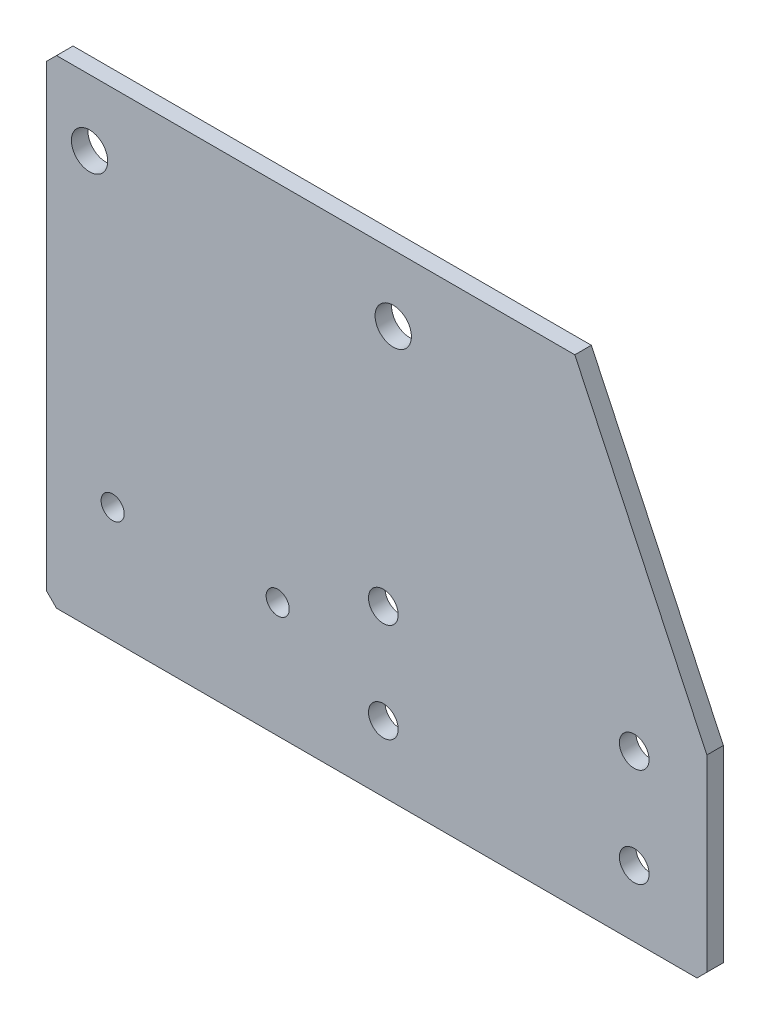
SolidWorks part; units mm, degrees
material "1023 碳钢板 (SS)"
ref_plane "前视基准面" through (0, 0, 0) normal (0, 0, 1) x (1, 0, 0)
ref_plane "上视基准面" through (0, 0, 0) normal (0, 1, 0) x (1, 0, 0)
ref_plane "右视基准面" through (0, 0, 0) normal (1, 0, 0) x (0, 0, -1)
ref_plane "基准面4" through (0, 0, 2.5) normal (0, 0, 1) x (1, 0, 0)
sketch "草图1" plane through (0, 0, 2.5) normal (0, 0, 1) x (1, 0, 0)
  line L0 (-97, -72.5) -> (97, -72.5)
  line L1 (97, -72.5) -> (100, -69.5)
  line L2 (100, -69.5) -> (100, -12.5)
  line L3 (100, -12.5) -> (60, 72.5)
  line L4 (60, 72.5) -> (-97, 72.5)
  line L5 (-97, 72.5) -> (-100, 69.5)
  line L6 (-100, 69.5) -> (-100, -69.5)
  line L7 (-100, -69.5) -> (-97, -72.5)
  circle A0 centre (2, -22.5) radius 4.5
  circle A1 centre (-30, -37.5) radius 3.5
  circle A2 centre (-80, -37.5) radius 3.5
  circle A3 centre (5, 52.5) radius 5.5
  circle A4 centre (78, -52.5) radius 4.5
  circle A5 centre (2, -52.5) radius 4.5
  circle A6 centre (78, -22.5) radius 4.5
  circle A7 centre (-87, 52.5) radius 5.5
extrude "凸台-拉伸1" add sketch "草图1" against normal blind 5
